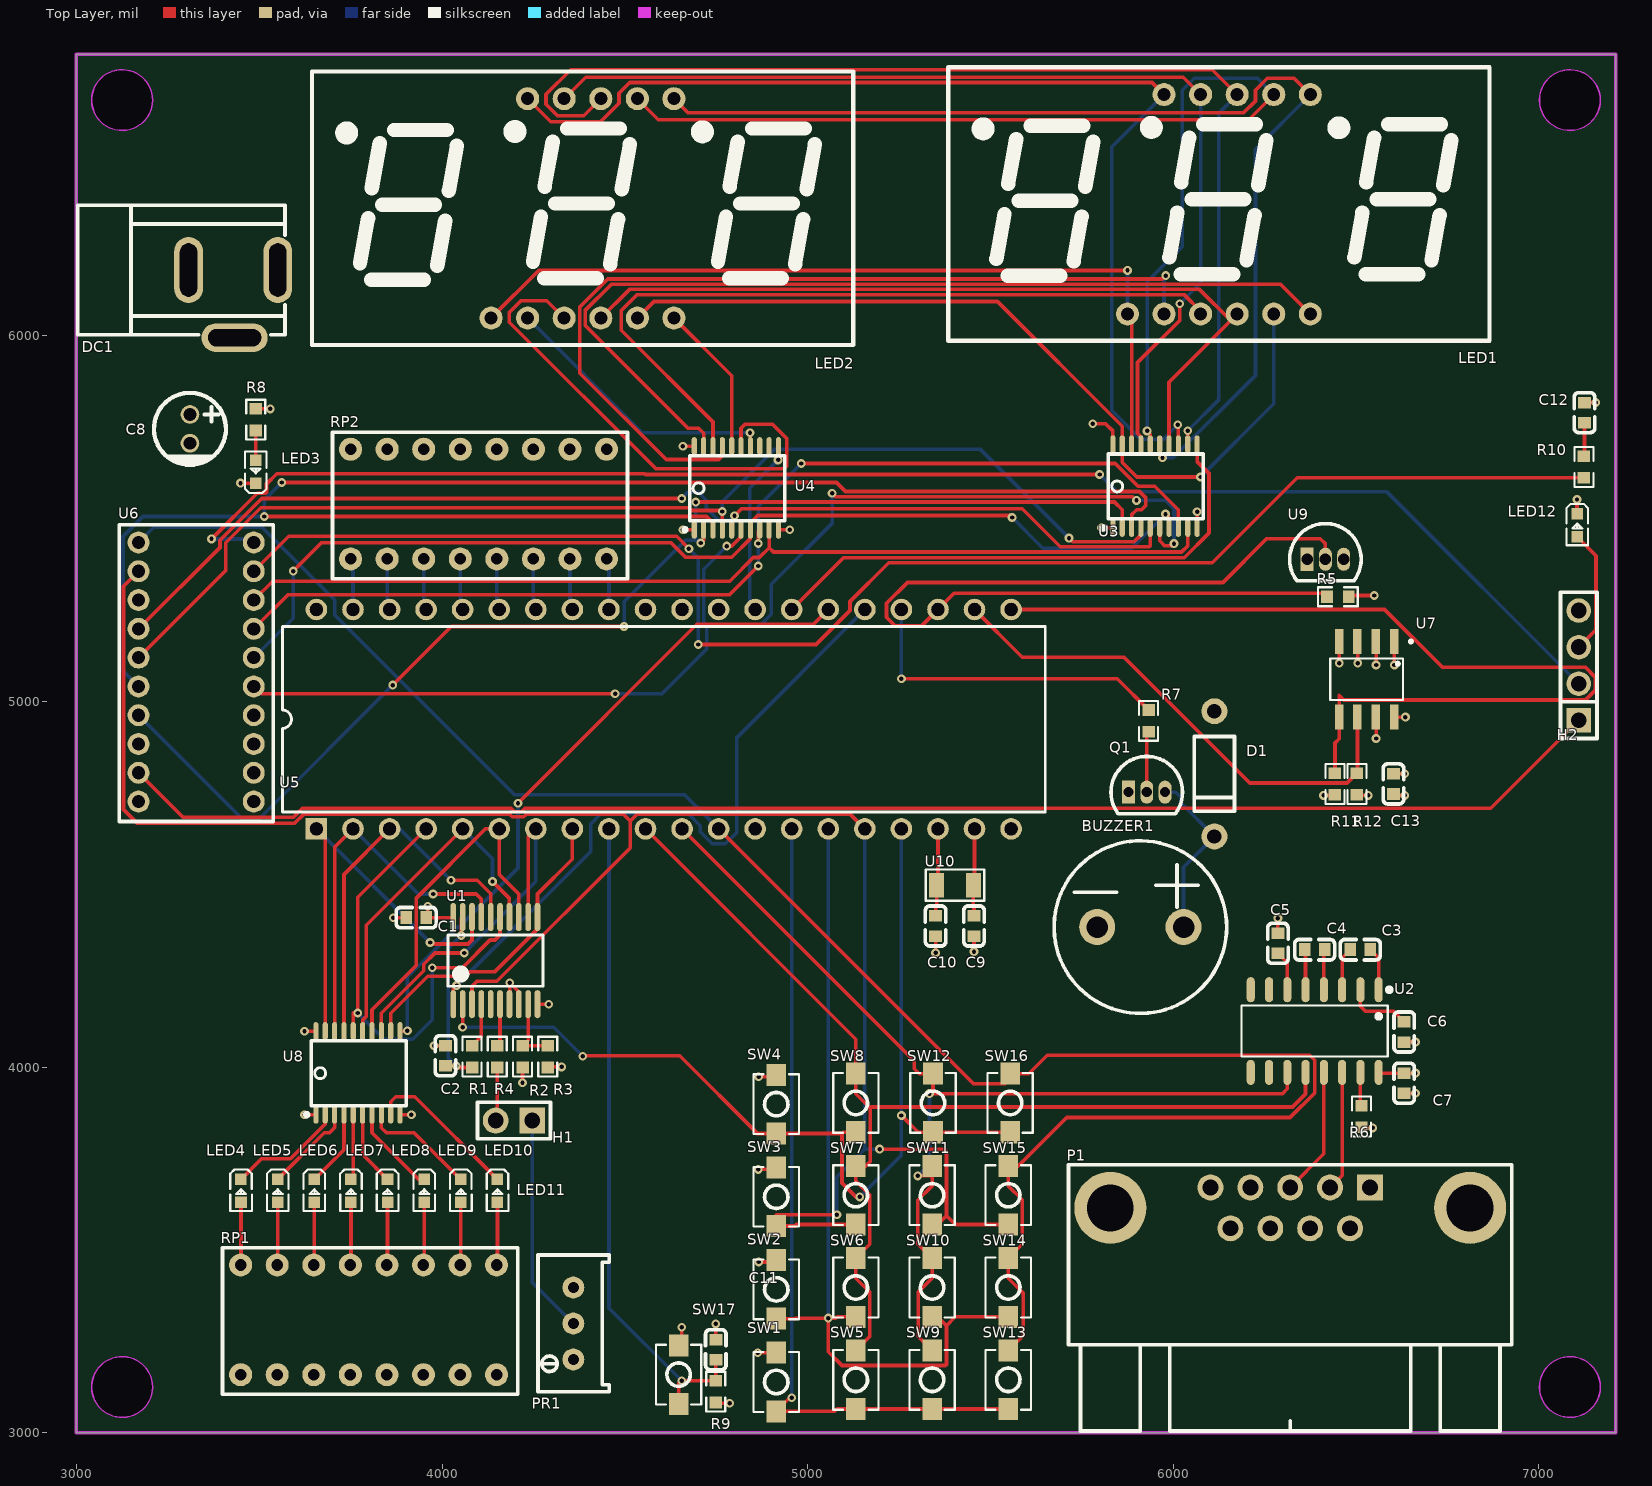
[diagram p0: Top Layer view]
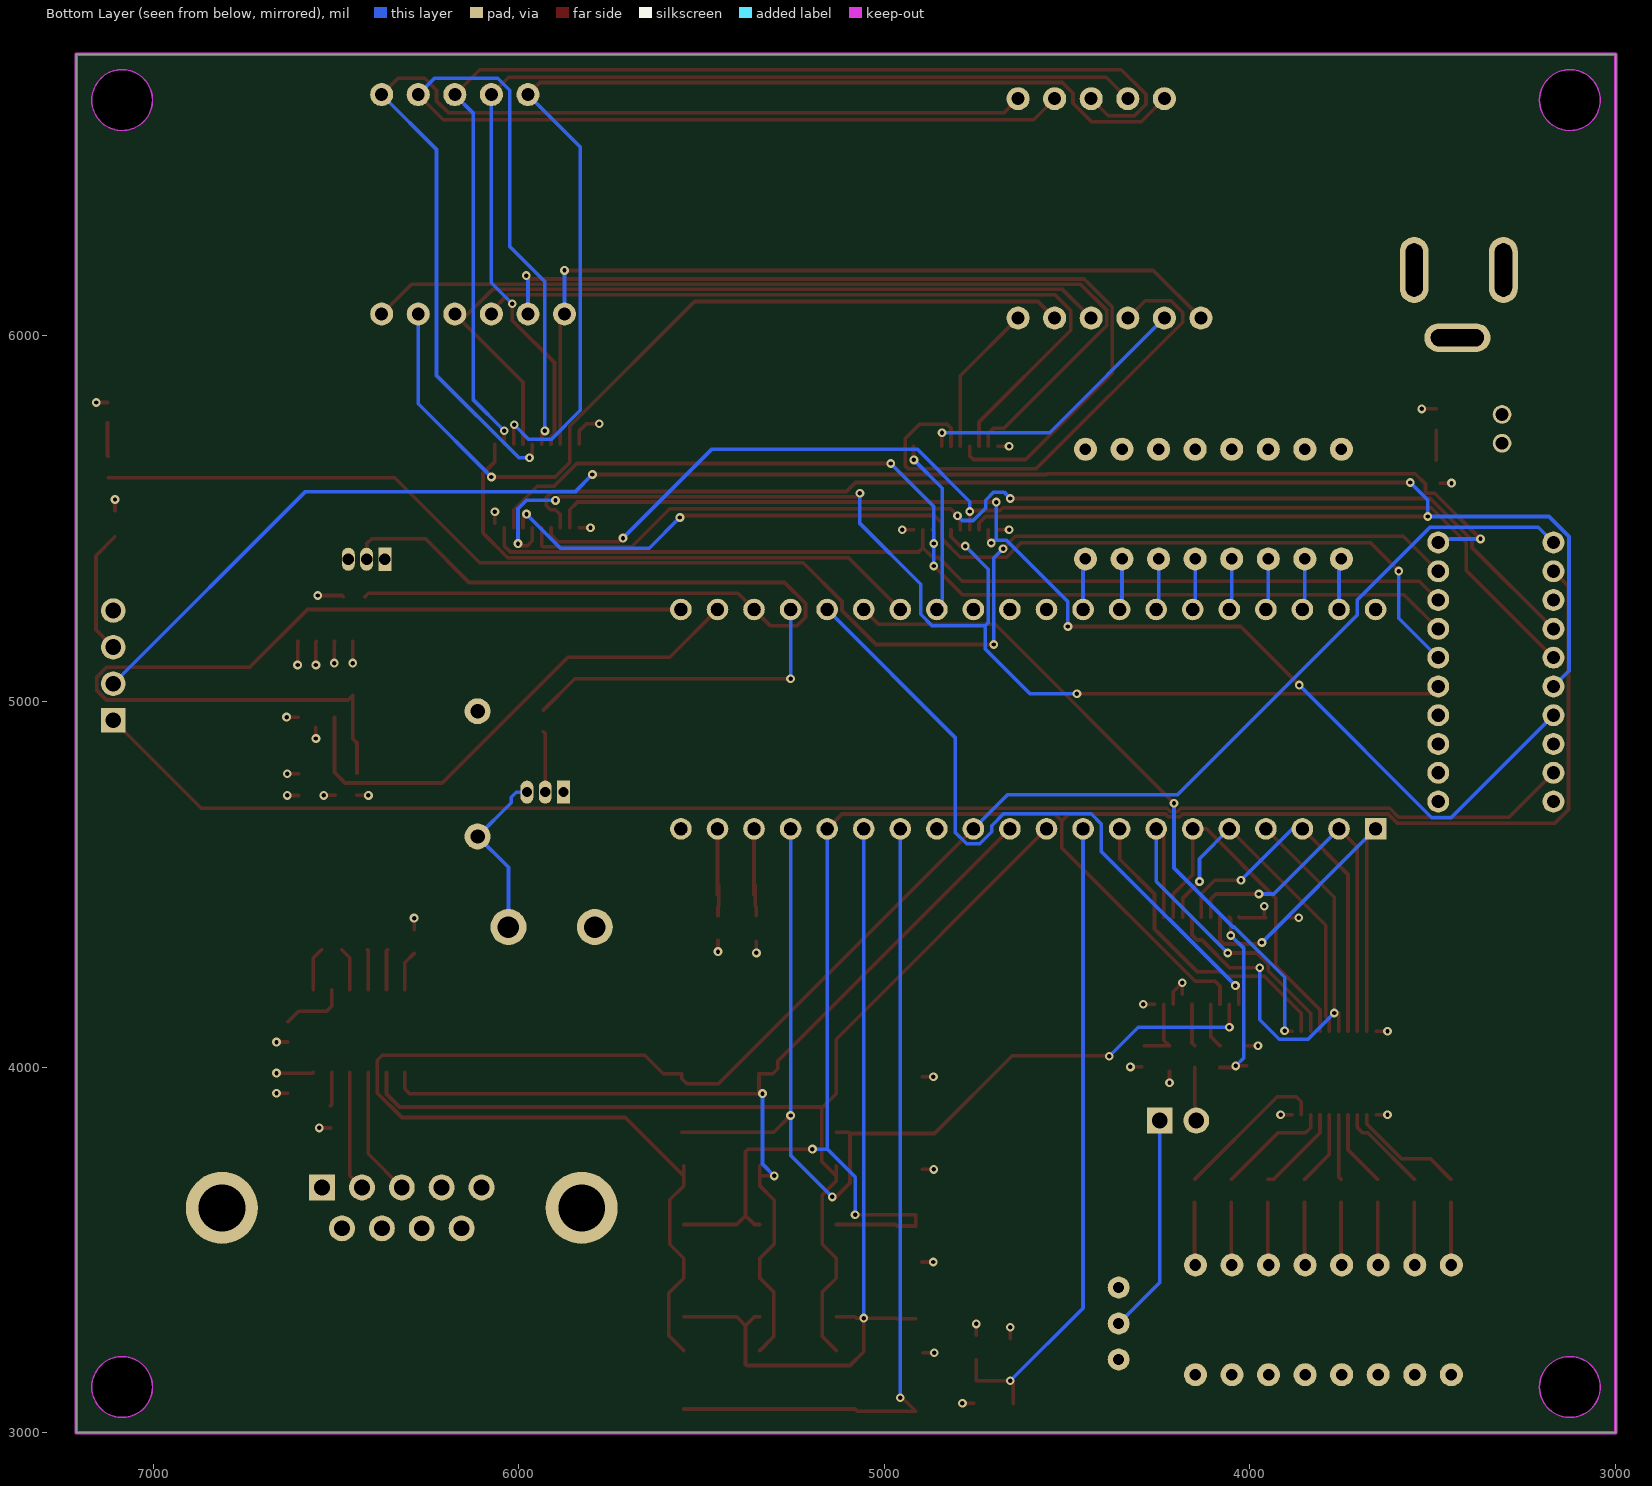
[diagram p1: Bottom Layer view, seen from below]
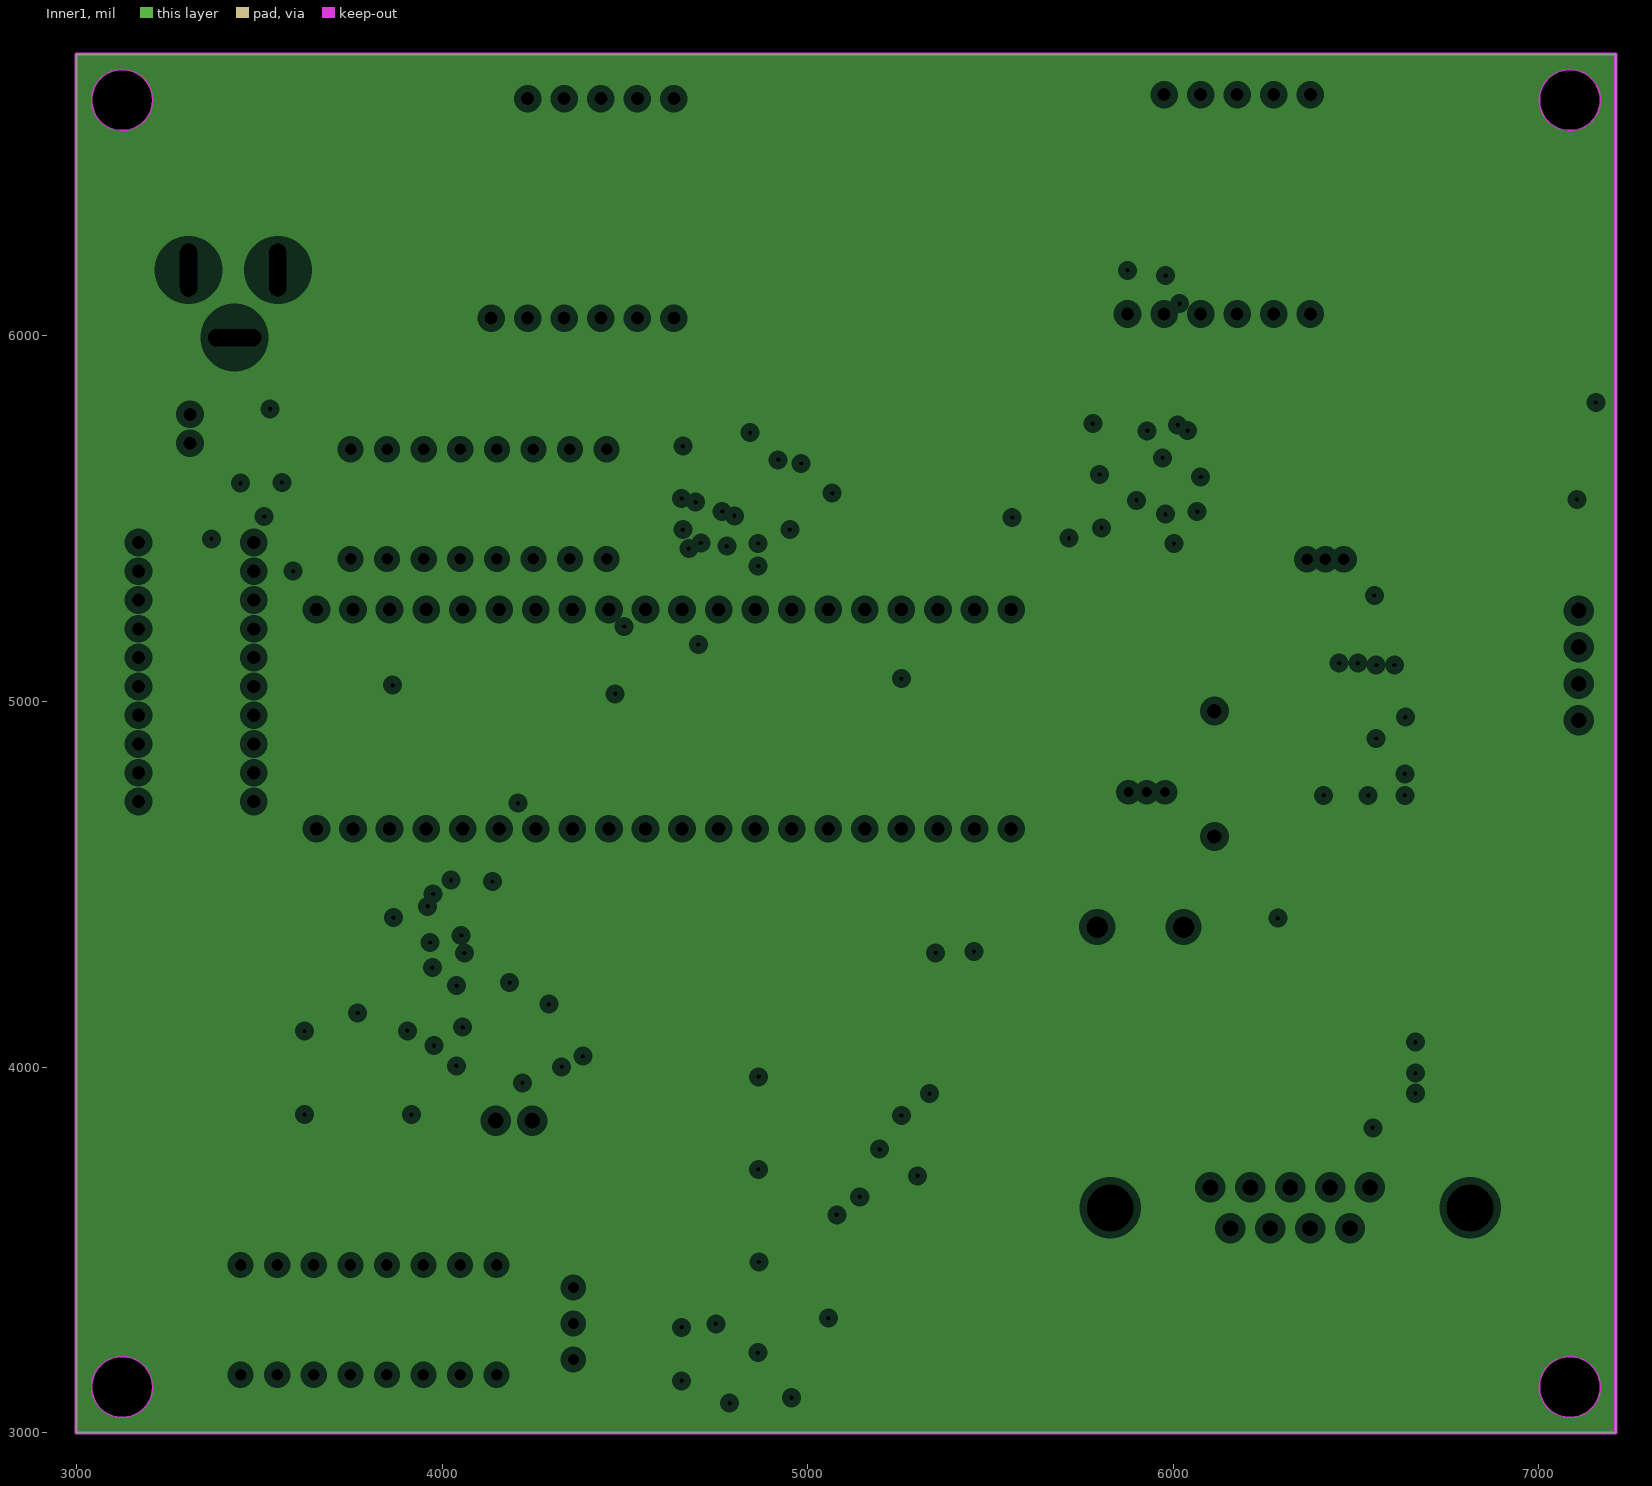
[diagram p2: Inner1, clearances drawn from the general rule]
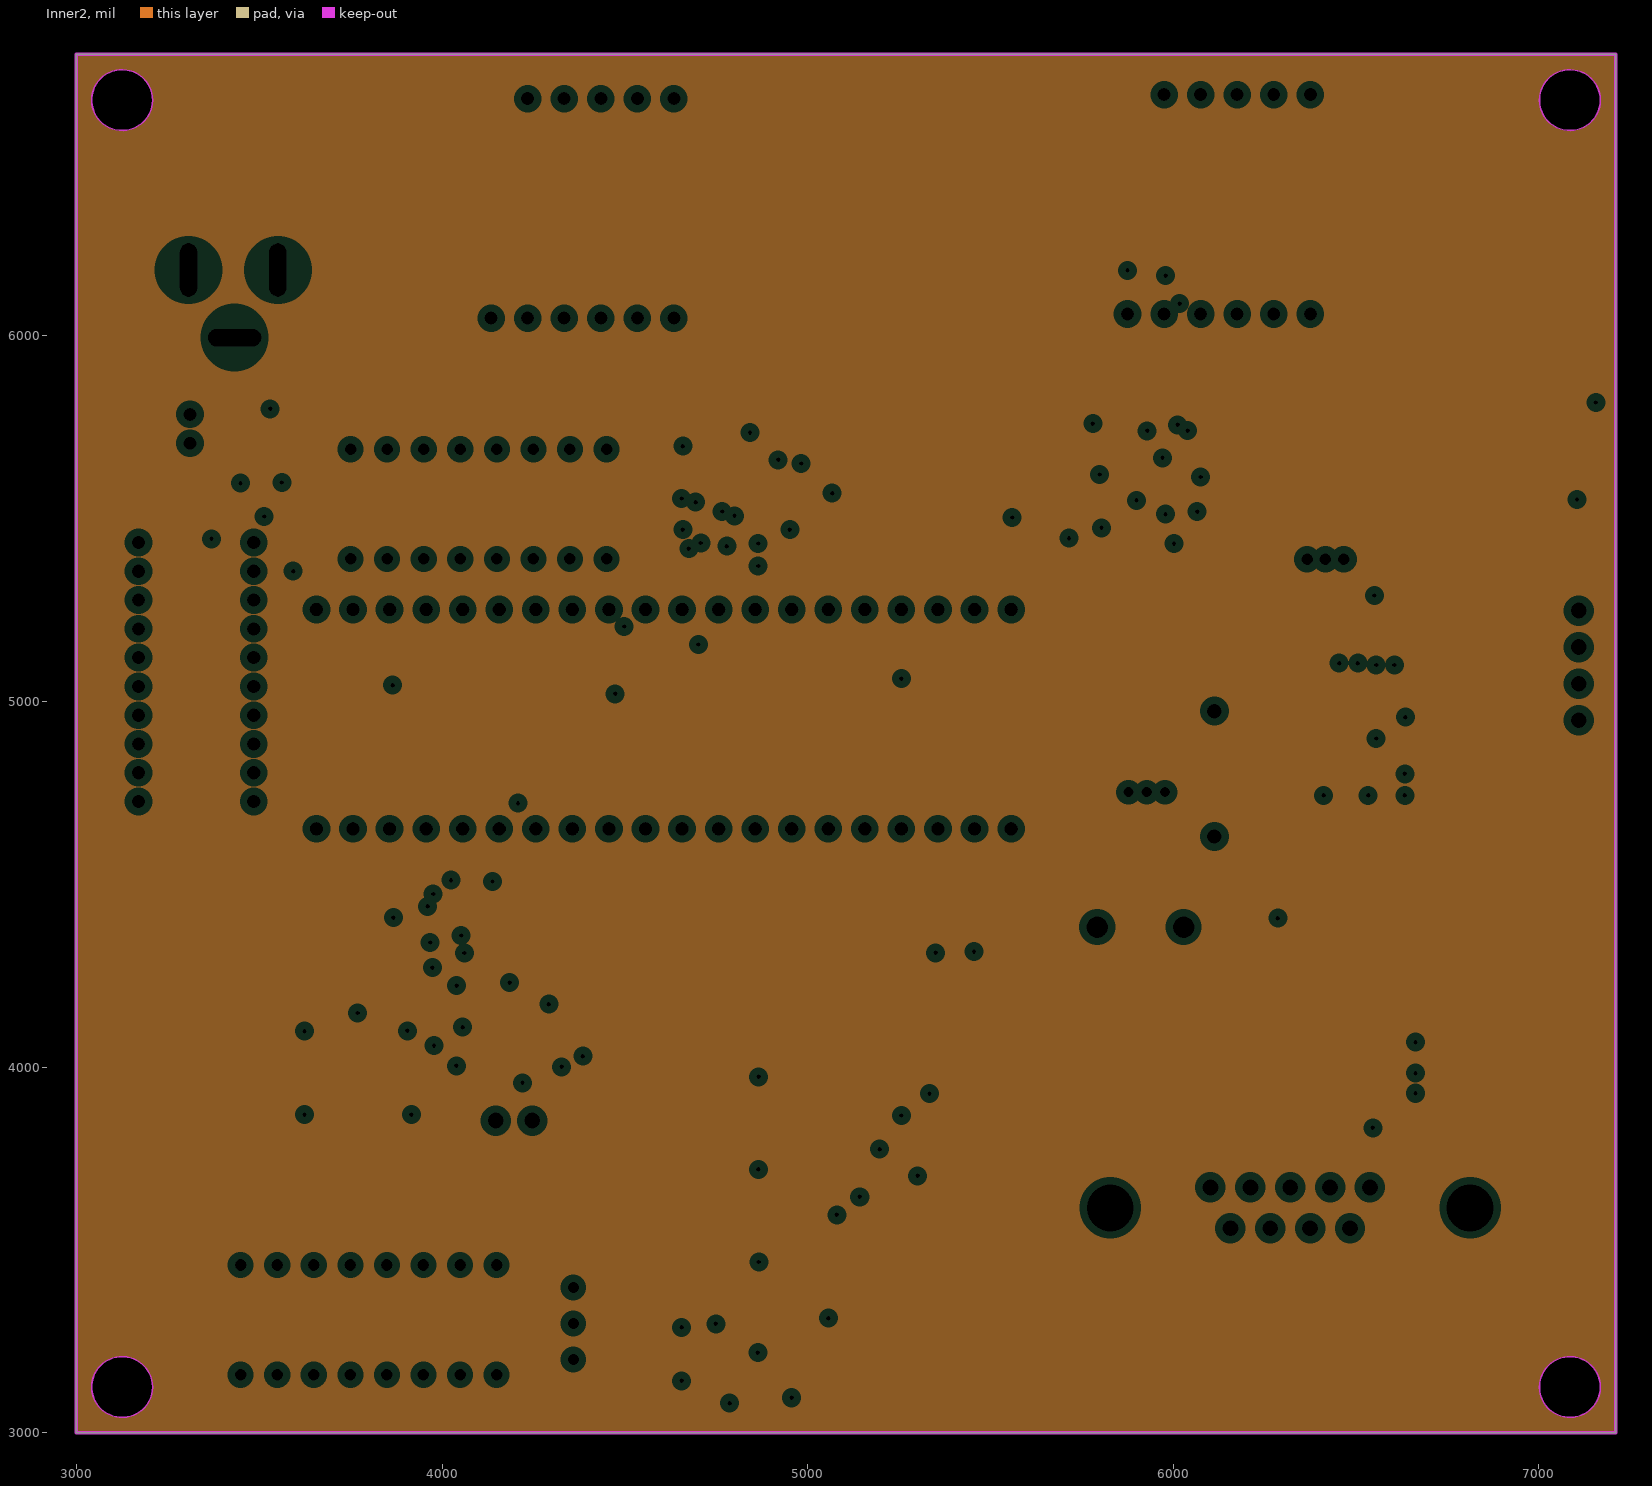
[diagram p3: Inner2, clearances drawn from the general rule]
# Altium PCB MISC49866.pcbdoc (part 1 of 2)
Units mil, origin at the board's own origin, x right, y up, seen from the top; angles counter-clockwise.
Board outline 4210 x 3770 mil, 4 copper layers (Top Layer, Inner1, Inner2, Bottom Layer), stack 62.447 mil thick; 74 components, 100 nets, 357 pads, 104 vias.

## Layer stack, top to bottom
Top Layer: signal copper 1.378
Dielectric1: surface 8.283, 7628 RC49% 8.6mil, Dk 4.4
Inner1: plane copper 0.598
Dielectric2: surface 41.929, 1.1mm H/HOZ Copper, Dk 4.43
Inner2: plane copper 0.598
Dielectric3: surface 8.283, 7628 RC49% 8.6mil, Dk 4.4
Bottom Layer: signal copper 1.378

## Board outline
3000,6770 3000,3000 7210,3000 7210,6770
cut-out: 3208.22,6645 cw(c3125,6645) 3041.78,6645 cw(c3125,6645)
cut-out: 7168.22,6645 cw(c7085,6645) 7001.78,6645 cw(c7085,6645)
cut-out: 7168.22,3125 cw(c7085,3125) 7001.78,3125 cw(c7085,3125)
cut-out: 3208.22,3125 cw(c3125,3125) 3041.78,3125 cw(c3125,3125)

## Design rules (kind name [scope] priority, off if disabled: settings)
BoardOutlineClearance copperThickness2oz_1 [All] p2 off: genericclearance=7.99 ignorepadtopadclearanceinfootprint=FALSE except(0: Arc-SplitContinuation Track-SplitContinuation SMDPad-SplitContinuation THPad-SplitContinuation Via-SplitContinuation Fill-SplitContinuation Region-SplitContinuation Poly-SplitContinuation Text-SplitContinuation Hole-SplitContinuation; 5.98: Arc-CutoutEdge SMDPad-CutoutEdge THPad-CutoutEdge Via-CutoutEdge Fill-CutoutEdge Region-CutoutEdge Text-CutoutEdge; 6.93: Hole-OutlineEdge Hole-CutoutEdge; 10: Poly-OutlineEdge Poly-CutoutEdge; 11.81: Arc-OutlineEdge Track-OutlineEdge SMDPad-OutlineEdge THPad-OutlineEdge Via-OutlineEdge Fill-OutlineEdge Region-OutlineEdge Text-OutlineEdge Track-CutoutEdge)
BoardOutlineClearance copperThickness1oz_1 [All] p4: genericclearance=4.02 ignorepadtopadclearanceinfootprint=FALSE except(0: Arc-SplitContinuation Track-SplitContinuation SMDPad-SplitContinuation THPad-SplitContinuation Via-SplitContinuation Fill-SplitContinuation Region-SplitContinuation Poly-SplitContinuation Text-SplitContinuation Hole-SplitContinuation; 6: SMDPad-CutoutEdge THPad-CutoutEdge Via-CutoutEdge Fill-CutoutEdge Region-CutoutEdge Text-CutoutEdge; 6.93: Hole-OutlineEdge Hole-CutoutEdge; 10: Poly-OutlineEdge Poly-CutoutEdge; 11.8: Arc-OutlineEdge Track-OutlineEdge SMDPad-OutlineEdge THPad-OutlineEdge Via-OutlineEdge Fill-OutlineEdge Region-OutlineEdge Text-OutlineEdge; 11.81: Arc-CutoutEdge Track-CutoutEdge)
Clearance copperThickness2oz [All] p1 off: gap=7.99 ignorepadtopadclearanceinfootprint=FALSE except(5.98: SMDPad-Track SMDPad-SMDPad THPad-Track SMDPad-THPad THPad-THPad Track-Via SMDPad-Via THPad-Via Via-Via Fill-Track Region-Track Fill-SMDPad Region-SMDPad Fill-THPad Region-THPad Fill-Via Region-Via Fill-Fill Fill-Region Region-Region Arc-Track Arc-SMDPad Arc-THPad Arc-Via Fill-Arc Region-Arc Arc-Arc Text-Track SMDPad-Text Text-THPad Text-Via Fill-Text Region-Text Arc-Text Text-Text; 6.93: Hole-Track Hole-SMDPad Hole-THPad Hole-Via Fill-Hole Region-Hole Hole-Arc Hole-Text; 10: Poly-Track Poly-SMDPad Poly-THPad Poly-Via Poly-Fill Poly-Region Poly-Poly Poly-Arc Poly-Text Poly-Hole)
Clearance copperThickness1oz [All] p3: gap=4.02 ignorepadtopadclearanceinfootprint=FALSE except(5.98: SMDPad-Track SMDPad-SMDPad THPad-Track SMDPad-THPad THPad-THPad Track-Via SMDPad-Via THPad-Via Via-Via Fill-Track Region-Track Fill-SMDPad Region-SMDPad Fill-THPad Region-THPad Fill-Via Region-Via Fill-Fill Fill-Region Region-Region; 6: Arc-Track Arc-SMDPad Arc-THPad Arc-Via Fill-Arc Region-Arc Arc-Arc Text-Track SMDPad-Text Text-THPad Text-Via Fill-Text Region-Text Arc-Text Text-Text; 6.93: Hole-Track Hole-SMDPad Hole-THPad Hole-Via Fill-Hole Region-Hole Hole-Arc Hole-Text; 10: Poly-Track Poly-SMDPad Poly-THPad Poly-Via Poly-Fill Poly-Region Poly-Poly Poly-Arc Poly-Text Poly-Hole)
Creepage creepage [All] p1: checkdistance=0 ignoreinternallayers=TRUE applytopolygonpour=TRUE
DiffPairsRouting differentialPair [All] p1: maxlimit=6 minlimit=6 mostfreqgap=6 toplayer_minwidth=5 toplayer_prefwidth=10 toplayer_maxwidth=100 toplayer_mingap=6 toplayer_prefgap=6 toplayer_maxgap=6 bottomlayer_minwidth=5 bottomlayer_prefwidth=10 bottomlayer_maxwidth=100 bottomlayer_mingap=6 bottomlayer_prefgap=6 bottomlayer_maxgap=6 maxuncoupledlength=10
HoleToHoleClearance otherClearance [All] p1: gap=11.81 allowstackedmicrovias=TRUE
Length netLength [All] p1: minlimit=0 maxlimit=0
MatchedLengths netLengthTolerance [All] p1: tolerance=1000
PasteMaskExpansion pasteMaskExpansion [All] p1: expansion=0
PlaneConnect innerPlane [All] p1: planeconnectstyle=Relief reliefexpansion=20 reliefentries=4 reliefconductorwidth=10 reliefairgap=10
PolygonConnect copperRegion [All] p1: connectstyle=Relief reliefconductorwidth=10 reliefentries=4 polygonreliefangle="90 Angle" airgapwidth=10 via.connectstyle=Relief via.reliefconductorwidth=10 via.reliefentries=4 via.polygonreliefangle="90 Angle" via.airgapwidth=10
RoutingVias viaSize [All] p1: holewidth=12.01 width=24.02 viastyle="Through Hole" minholewidth=11.81 minwidth=19.68 maxholewidth=248.03 maxwidth=393.7
SolderMaskExpansion solderMaskExpansion [IsVia] p1: expansion=-1000 istentingtop=TRUE
SolderMaskExpansion solderMaskExpansion [All] p2: expansion=2 istentingtop=FALSE
Width copperThickness2oz_2 [All] p1 off: maxlimit=100 minlimit=8 preferedwidth=10
Width PWR [(InNet('VCC'))] p2: maxlimit=10 minlimit=10 preferedwidth=10 toplayer_minwidth=10 toplayer_maxwidth=100 toplayer_prefwidth=30 bottomlayer_minwidth=10 bottomlayer_maxwidth=100 bottomlayer_prefwidth=30
Width copperThickness1oz_2 [All] p3: maxlimit=10 minlimit=10 preferedwidth=10 toplayer_minwidth=10 toplayer_maxwidth=100 toplayer_prefwidth=10 bottomlayer_minwidth=10 bottomlayer_maxwidth=100 bottomlayer_prefwidth=10

## Components (designator, comment, footprint, x,y, rotation, side; value= is the part's Value field where it differs from the comment)
BUZZER1 "buzzer" BUZ-TH_BD12.0-P6.00-D0.9-RD 5910.16,4383.1 r0 top
C1 "104" C0603 3929.27,4408.78 r180 top
C2 "104" C0603 4009.27,4030.97 r90 top
C3 "104" C0603 6511.76,4321.11 r180 top
C4 "104" C0603 6386.76,4321.11 r180 top
C5 "104" C0603 6286.36,4338.55 r270 top
C6 "104" C0603 6631.76,4096.11 r90 top
C7 "104" C0603 6631.76,3956.11 r90 top
C8 "100uF" CAP-TH_BD5.0-P2.00-D0.8-FD-10UF50VC110GL 3310.61,5745.83 r270 top
C9 "20PF" C0603 5455.03,4386.04 r90 top
C10 "20PF" C0603 5350.03,4386.04 r90 top
C11 "10uF" C0603 4748.84,3227.23 r90 top
C12 "104" C0603 7124.88,5790.25 r90 top
C13 "104" C0603 6602.32,4774.62 r270 top
D1 "" DO_1N4007 6112.67,4802.17 r90 top
DC1 "" DC-005_2.5 3423.86,6167.74 r180 top
H1 "" HDR-TH_2P-P2.54-V-M-1 4196.93,3853.78 r180 top
H2 "" HDR-TH_4P-P2.54-V-M 7109.27,5098.78 r90 top
LED1 "3631BS" LED-SEG-TH_11P-L37.5-W19.0-P2.54-LS15.2-BL_1 6125,6360 r180 top
LED2 "3631BS" LED-SEG-TH_11P-L37.5-W19.0-P2.54-LS15.2-BL_1 4384.27,6348.78 r180 top
LED3 "" LED_0603 3490.61,5630.83 r90 top
LED4 "" LED_0603 3450.42,3659.36 r270 top
LED5 "" LED_0603 3550.64,3659.36 r270 top
LED6 "" LED_0603 3650.86,3659.36 r270 top
LED7 "" LED_0603 3751.08,3659.36 r270 top
LED8 "" LED_0603 3851.3,3659.36 r270 top
LED9 "" LED_0603 3951.52,3659.36 r270 top
LED10 "" LED_0603 4051.73,3659.36 r270 top
LED11 "" LED_0603 4151.95,3659.36 r270 top
LED12 "" LED_0603 7105,5480 r270 top
P1 "DB9FL" DB9-TH_DB9F 6320,3615 r0 top
PR1 "10kΩ" R_3296 4354.27,3298.78 r90 top
Q1 "" S8550P_TO-92 5927.67,4752.17 r0 top
R1 "10K" R0603 4082.23,4028.78 r90 top
R2 "1K" R0603 4220.26,4028.78 r270 top
R3 "1K" R0603 4289.27,4028.78 r90 top
R4 "510K" R0603 4151.25,4028.78 r90 top
R5 "4.7K" R0603 6450.25,5286.78 r0 top
R6 "0" R0603 6515,3865 r90 top
R7 "2K" R0603 5932.67,4947.17 r270 top
R8 "1K" R0603 3490.61,5770.83 r90 top
R9 "10K" R0603 4748.84,3112.23 r90 top
R10 "0" R0603 7123.25,5641.69 r90 top
R11 "4.7K" R0603 6442.32,4774.62 r270 top
R12 "4.7K" R0603 6502.32,4774.62 r270 top
RP1 "" DIP-16_L20.3-W10.2-P2.54-LS7.6-BL 3799.27,3308.78 r0 top
RP2 "" DIP-16_L20.3-W10.2-P2.54-LS7.6-BL 4100,5540 r0 top
SW1 "" Key_SMD_3x4x2 4914.27,3138.78 r270 top
SW2 "" Key_SMD_3x4x2 4914.27,3392.12 r270 top
SW3 "" Key_SMD_3x4x2 4914.27,3645.45 r270 top
SW4 "" Key_SMD_3x4x2 4914.27,3898.78 r270 top
SW5 "" Key_SMD_3x4x2 5131.95,3144.87 r90 top
SW6 "" Key_SMD_3x4x2 5131.95,3397.24 r90 top
SW7 "" Key_SMD_3x4x2 5131.95,3649.62 r90 top
SW8 "" Key_SMD_3x4x2 5131.95,3901.99 r90 top
SW9 "" Key_SMD_3x4x2 5340.44,3144.87 r90 top
SW10 "" Key_SMD_3x4x2 5340.44,3397.24 r90 top
SW11 "" Key_SMD_3x4x2 5340.44,3649.62 r90 top
SW12 "" Key_SMD_3x4x2 5342.94,3901.99 r90 top
SW13 "" Key_SMD_3x4x2 5548.93,3144.87 r90 top
SW14 "" Key_SMD_3x4x2 5548.93,3397.24 r90 top
SW15 "" Key_SMD_3x4x2 5548.93,3649.62 r90 top
SW16 "" Key_SMD_3x4x2 5553.93,3901.99 r90 top
SW17 "" Key_SMD_3x4x2 4647.12,3159.02 r270 top
U1 "ADC0804CN" ADC0804CN 4131,4303.28 r0 top
U2 "MAX232ESE" MAX232ESE 6591.76,4211.11 r180 top
U3 "MC74HC573DW" MC74HC573DW 5835,5475 r90 top
U4 "MC74HC573DW" MC74HC573DW 4690,5470 r90 top
U5 "P89C51RC2HBP" P89C51RC23N_01 4754.31,4907.16 r0 top
U6 "DAC0832LCJ" DAC0832LCJ 3485,5435 r0 top
U7 "AT24C02" SOIC-8_L5.0-W4.0-P1.27-LS6.2-TL 6528.96,5060.68 r270 top
U8 "MC74HC573DW" MC74HC573DW 3655,3870 r90 top
U9 "DS18B20" TO-92-3_L4.9-W3.7-P1.27-L 6416.26,5389.12 r0 top
U10 "32768/10ppm/12.5pF" osc-smd_l3.2-w1.5 5403.24,4497.68 r0 top

## Footprints (in the part's own frame and the unit in brackets; to place one, negate y for a bottom-side part, rotate by r counter-clockwise, add the part's x,y. Pads: shape width x height; smd on the part's side, far side on the other; paste and mask are expansions set on the pad)
ADC0804CN [mm]
  oval 0.4x1.95 smd: 1(-2.544,-3.334) 2(-1.894,-3.334) 3(-1.244,-3.334) 4(-0.594,-3.334) 5(0.056,-3.334) 6(0.706,-3.334) 7(1.356,-3.334) 8(2.006,-3.334) 9(2.656,-3.334) 10(3.306,-3.334) 11(3.306,2.724) 12(2.656,2.724) 13(2.006,2.724) 14(1.356,2.724) 15(0.706,2.724) 16(0.056,2.724) 17(-0.594,2.724) 18(-1.244,2.724) 19(-1.894,2.724) 20(-2.544,2.724)
  silkscreen extent -2.92,-2.08 3.68,1.47
BUZ-TH_BD12.0-P6.00-D0.9-RD [mm]
  round 2.5 hole 1.5 paste+0 mask+0.05: 1(-3,0) 2(3,0)
  silkscreen extent -5.99,-5.99 5.99,5.99
C0603 [mm]
  rect 0.8x0.9 smd: 1(-0.7,0) 2(0.7,0)
  silkscreen extent -1.39,-0.71 1.39,0.71
CAP-TH_BD5.0-P2.00-D0.8-FD-10UF50VC110GL [mm]
  round 1.3 hole 0.9 paste+0 mask+0.051: 1(-1,0) 2(1,0)
  silkscreen extent -2.5,-2.5 2.5,2.5
DAC0832LCJ [mil]
  round 60 hole 36 paste+0 mask+2: 1(-314.96,0) 2(-314.96,-78.74) 3(-314.96,-157.48) 4(-314.96,-236.22) 5(-314.96,-314.96) 6(-314.96,-393.7) 7(-314.96,-472.44) 8(-314.96,-551.18) 9(-314.96,-629.92) 10(-314.96,-708.66) 11(0,0) 12(0,-78.74) 13(0,-157.48) 14(0,-236.22) 15(0,-314.96) 16(0,-393.7) 17(0,-472.44) 18(0,-551.18) 19(0,-629.92) 20(0,-708.66)
  silkscreen extent -368,-763 53,49
DB9-TH_DB9F [mm]
  rect 1.8x1.8 hole 1.1: 1(5.54,1.42)
  round 1.8 hole 1.1: 2(2.77,1.42) 3(0,1.42) 4(-2.77,1.42) 5(-5.54,1.42) 6(4.155,-1.42) 7(1.385,-1.42) 8(-1.385,-1.42) 9(-4.155,-1.42)
  round 5 hole 3.25: 10(-12.5,0) 11(12.5,0)
  silkscreen extent -15.4,-15.5 15.4,3
DC-005_2.5 [mm]
  oval 2x4.6 hole 1.2 slot 3.7 at 90 deg paste+0 mask+0.051: 1(-3.227,-0.318) 2(2.973,-0.318)
  oval 4.6x2 hole 1.2 slot 3.7 at 0 deg paste+0 mask+0.051: 3(-0.227,4.382)
  silkscreen extent -3.73,-4.82 10.67,4.18
DIP-16_L20.3-W10.2-P2.54-LS7.6-BL [mm]
  round 1.6 hole 0.8: 1(-8.89,-3.81) 2(-6.35,-3.81) 3(-3.81,-3.81) 4(-1.27,-3.81) 5(1.27,-3.81) 6(3.81,-3.81) 7(6.35,-3.81) 8(8.89,-3.81) 9(8.89,3.81) 10(6.35,3.81) 11(3.81,3.81) 12(1.27,3.81) 13(-1.27,3.81) 14(-3.81,3.81) 15(-6.35,3.81) 16(-8.89,3.81)
  silkscreen extent -10.15,-5.18 10.35,5
DO_1N4007 [mm]
  round 1.8 hole 1 paste+0 mask+0.051: 1(-4.35,0) 2(4.35,0)
  silkscreen extent -2.6,-1.4 2.6,1.4
HDR-TH_2P-P2.54-V-M-1 [mm]
  rect 1.8x1.8 hole 1.1: 1(-1.27,0)
  round 1.8 hole 1.1: 2(1.27,0)
  silkscreen extent -2.54,-1.27 2.54,1.27
HDR-TH_4P-P2.54-V-M [mm]
  rect 1.7x1.7 hole 1.1: 1(-3.81,0)
  round 1.7 hole 1.1: 2(-1.27,0) 3(1.27,0) 4(3.81,0)
  silkscreen extent -5.08,-1.27 5.08,1.27
Key_SMD_3x4x2 [mm]
  rect 1.53x1.36 smd paste+0 mask+0.051: 1(-2.035,0) 2(2.035,0)
  silkscreen extent -2.08,-1.58 2.08,1.58
LED-SEG-TH_11P-L37.5-W19.0-P2.54-LS15.2-BL_1 [mm]
  round 1.6 hole 0.9: 1(-6.35,-7.62) 2(-3.81,-7.62) 3(-1.27,-7.62) 4(1.27,-7.62) 5(3.81,-7.62) 7(6.35,7.62) 8(3.81,7.62) 9(1.27,7.62) 10(-1.27,7.62) 11(-3.81,7.62) 12(-6.35,7.62)
  silkscreen extent -18.8,-9.51 18.8,9.49
LED_0603 [mil]
  rect 31.5x31.5 smd paste+0 mask+2: 1(-33.5,-0.4) 2(29.5,-0.2)
  silkscreen extent -61,-30 53,30
MAX232ESE [mm]
  oval 0.56x1.745 smd paste+0.102 mask+0.051: 1(0.755,-0.016) 2(2.025,-0.016) 3(3.295,-0.016) 4(4.565,-0.016) 5(5.835,-0.016) 6(7.105,-0.016) 7(8.375,-0.016) 8(9.645,-0.016) 9(9.645,5.728) 10(8.375,5.728) 11(7.105,5.728) 12(5.835,5.728) 13(4.565,5.728) 14(3.295,5.728) 15(2.025,5.728) 16(0.755,5.728)
  silkscreen extent -0.13,-0.17 10.28,4.63
MC74HC573DW [mm]
  oval 1.26x0.36 smd: 1(0,0) 2(0,-0.65) 3(0,-1.3) 4(0,-1.95) 5(0,-2.6) 6(0,-3.25) 7(0,-3.9) 8(0,-4.55) 9(0,-5.2) 10(0,-5.85) 11(5.8,-5.85) 12(5.8,-5.2) 13(5.8,-4.55) 14(5.8,-3.9) 15(5.8,-3.25) 16(5.8,-2.6) 17(5.8,-1.95) 18(5.8,-1.3) 19(5.8,-0.65) 20(5.8,0)
  silkscreen extent -0.05,-6.27 5.13,0.68
osc-smd_l3.2-w1.5 [mm]
  rect 1.05x1.7 smd: 1(-1.275,0) 2(1.275,0)
  silkscreen extent -2.03,-1.08 2.03,1.08
P89C51RC23N_01 [mm]
  rect 1.5x1.5 hole 0.9 slot 0.905 at 90 deg paste+0 mask+0.051: 1(-27.883,-6.489)
  round 1.5 hole 0.9 slot 0.905 at 90 deg paste+0 mask+0.051: 2(-25.343,-6.489) 3(-22.803,-6.489) 4(-20.263,-6.489) 5(-17.723,-6.489) 6(-15.183,-6.489) 7(-12.643,-6.489) 8(-10.103,-6.489) 9(-7.563,-6.489) 10(-5.023,-6.489) 11(-2.483,-6.489) 12(0.057,-6.489) 13(2.597,-6.489) 14(5.137,-6.489) 15(7.677,-6.489) 16(10.217,-6.489) 17(12.757,-6.489) 18(15.297,-6.489) 19(17.837,-6.489) 20(20.377,-6.489) 21(20.377,8.751) 22(17.837,8.751) 23(15.297,8.751) 24(12.757,8.751) 25(10.217,8.751) 26(7.677,8.751) 27(5.137,8.751) 28(2.597,8.751) 29(0.057,8.751) 30(-2.483,8.751) 31(-5.023,8.751) 32(-7.563,8.751) 33(-10.103,8.751) 34(-12.643,8.751) 35(-15.183,8.751) 36(-17.723,8.751) 37(-20.263,8.751) 38(-22.803,8.751) 39(-25.343,8.751) 40(-27.883,8.751)
  silkscreen extent -30.25,-5.32 22.75,7.58
R0603 [mil]
  rect 31.75x34.02 smd paste-3937.01 mask+2: 1(-29.66,0) 2(29.66,0)
  silkscreen extent -55,-26 55,26
R_3296 [mil]
  round 60 hole 30 paste+0 mask+2: 1(-98.4,-5) 2(0,-5) 3(98.4,-5)
  silkscreen extent -187,-103 187,92
S8550P_TO-92 [mm]
  rect 0.9x1.6 hole 0.7 paste+0 mask+0.051: 1(-1.27,0)
  oval 0.9x1.6 hole 0.7 paste+0 mask+0.051: 2(0,0) 3(1.27,0)
  silkscreen extent -2.48,-1.5 2.48,2.48
SOIC-8_L5.0-W4.0-P1.27-LS6.2-TL [mil]
  rect 68.92x23.18 smd: 1(-103.36,75) 2(-103.36,25) 3(-103.36,-25) 4(-103.36,-75) 5(103.36,-75) 6(103.36,-25) 7(103.36,25) 8(103.36,75)
  silkscreen extent -107,-99 57,125
TO-92-3_L4.9-W3.7-P1.27-L [mm]
  rect 0.9x1.6 hole 0.8: 1(-1.27,0)
  oval 0.9x1.6 hole 0.8: 2(0,0) 3(1.27,0)
  silkscreen extent -2.48,-1.5 2.48,2.48

## Via types
v1: diameter 24.02, hole 12, Top Layer to Bottom Layer, 104 vias

## Nets (pads, with @x,y where several pads share a name; then routed paths per layer and width w, separated by ;. In a path a pad name is that pad's centre, name@x,y a point inside that pad or via, vN(x,y) a via of type N, cw(c..) or ccw(c..) an arc to the next point about the centre after c; other vN are vias at no path point)
18B20: R5.1 U5.23 U9.2 | length 2613.9
  Top Layer w10: U9.2@6416.26,5389.12 6416.26,5431.36 6402.49,5445.13 6255.24,5445.13 6135.86,5325.75 5273.08,5325.75 5215.87,5268.54 5215.87,5230.52 5238.67,5207.72 5312.59,5207.72 U5.23@5356.56,5251.69 5400.67,5295.8 6411.57,5295.8 R5.1@6420.59,5286.78
$1N14: R1.2 U1.4 | length 124.1
  Top Layer w10: R1.2@4082.23,4058.44 4107.62,4083.82 U1.4@4107.62,4172.03
$1N15: C2.1 R1.1 U1.19 | length 507.6
  Top Layer w10: C2.1@4009.27,4003.41 v1(4039.19,4003.41) 4043.48,3999.12 R1.1@4082.23,3999.12 ; v1(4052.37,4359.97) 4052.37,4406.46 U1.19@4056.44,4410.54
  Bottom Layer w10: v1(4039.19,4003.41) 4016.71,4025.89 4016.71,4324.31 v1(4052.37,4359.97)
$1N18: H1.1 PR1.2 | length 601.5
  Bottom Layer w10: H1.1@4246.93,3853.78 4246.93,3411.12 PR1.2@4359.27,3298.78
$1N20: R2.1 R3.2 U1.9 | length 189
  Top Layer w10: U1.9@4235.57,4172.03 4235.57,4073.76 R2.1@4220.26,4058.44 R3.2@4289.27,4058.44
$1N23: R4.2 U1.6 | length 116.7
  Top Layer w10: R4.2@4151.25,4058.44 4158.81,4066 U1.6@4158.8,4172.03
$1N24: H1.2 R4.1 | length 147.1
  Top Layer w10: H1.2@4146.93,3853.78 4151.25,3858.09 R4.1@4151.25,3999.12
$1N28: C3.1 U2.1 | length 118.8
  Top Layer w10: C3.1@6539.32,4321.11 6562.02,4298.41 U2.1@6562.02,4211.76
$1N29: C3.2 U2.3 | length 118.5
  Top Layer w10: U2.3@6462.02,4211.76 6462.02,4298.93 C3.2@6484.2,4321.11
$1N30: C4.2 U2.5 | length 110.5
  Top Layer w10: C4.2@6359.2,4321.11 6362.02,4318.29 U2.5@6362.02,4211.76
$1N31: C4.1 U2.4 | length 110.3
  Top Layer w10: U2.4@6412.02,4211.76 6412.02,4318.81 C4.1@6414.32,4321.11
$1N34: R6.2 U2.15 | length 92.2
  Top Layer w10: U2.15@6512.02,3985.58 6512.02,3897.64 R6.2@6515,3894.66
$1N36: P1.3 U2.13 | length 352.8
  Top Layer w10: P1.3@6320.01,3670.91 6412.02,3762.93 U2.13@6412.02,3985.58
$1N37: P1.2 U2.14 | length 328.3
  Top Layer w10: P1.2@6429.06,3670.91 6462.02,3703.87 U2.14@6462.02,3985.58
$1N38: C5.2 U2.6 | length 109.9
  Top Layer w10: C5.2@6286.35,4310.99 6312.02,4285.32 U2.6@6312.02,4211.76
$1N40: C6.2 U2.2 | length 182.6
  Top Layer w10: U2.2@6512.02,4211.76 6512.02,4166.68 6525.79,4152.91 6602.52,4152.91 C6.2@6631.76,4123.67
$1N109: BUZZER1.2 D1.1 Q1.3 | length 476.9
  Bottom Layer w10: Q1.3@5977.67,4752.17 6006.62,4752.17 6020.39,4738.4 6020.39,4723.19 D1.1@6112.67,4630.91 6028.28,4546.52 BUZZER1.2@6028.27,4383.1
$1N111: Q1.2 R7.2 | length 167.4
  Top Layer w10: Q1.2@5927.67,4752.17 5927.67,4912.51 R7.2@5932.67,4917.51
$1N114: LED3.2 R8.1 | length 80.9
  Top Layer w10: R8.1@3490.61,5741.17 3490.81,5740.96 LED3.2@3490.81,5660.33
$1N128: LED4.1 U8.2 | length 318.8
  Top Layer w10: LED4.1@3450.02,3692.86 3506.48,3749.31 3585.34,3749.31 3680.59,3844.56 U8.2@3680.59,3870
$1N129: LED5.1 U8.3 | length 250.1
  Top Layer w10: LED5.1@3550.24,3692.86 3678.08,3820.7 3692.41,3820.7 3706.18,3834.47 U8.3@3706.18,3870
$1N130: LED5.2 RP1.15 | length 171.6
  Top Layer w10: RP1.15@3549.27,3458.78 3550.44,3459.94 LED5.2@3550.44,3629.86
$1N131: LED7.2 RP1.13 | length 171.7
  Top Layer w10: RP1.13@3749.27,3458.78 3750.88,3460.38 LED7.2@3750.88,3629.86
$1N132: LED7.1 U8.5 | length 179.9
  Top Layer w10: LED7.1@3750.68,3692.86 3757.36,3699.54 U8.5@3757.36,3870
$1N133: LED6.1 U8.4 | length 210.8
  Top Layer w10: LED6.1@3650.46,3692.86 3731.77,3774.17 U8.4@3731.77,3870
$1N134: LED9.2 RP1.11 | length 171.9
  Top Layer w10: RP1.11@3949.27,3458.78 3951.32,3460.82 LED9.2@3951.32,3629.86
$1N135: LED9.1 U8.7 | length 244.8
  Top Layer w10: U8.7@3808.54,3870 3808.54,3820.7 3936.38,3692.86 LED9.1@3951.12,3692.86
$1N136: LED8.1 U8.6 | length 205.3
  Top Layer w10: U8.6@3782.95,3870 3782.95,3760.81 LED8.1@3850.9,3692.86
$1N137: LED11.2 RP1.9 | length 172.1
  Top Layer w10: RP1.9@4149.27,3458.78 4151.76,3461.26 LED11.2@4151.75,3629.86
$1N138: LED11.1 U8.9 | length 426.9
  Top Layer w10: U8.9@3859.72,3870 3859.72,3905.53 3873.49,3919.3 3925.12,3919.3 LED11.1@4151.55,3692.86
$1N139: LED10.1 U8.8 | length 311.4
  Top Layer w10: U8.8@3834.13,3870 3834.13,3834.47 3847.9,3820.7 3923.5,3820.7 LED10.1@4051.33,3692.86
$1N140: LED4.2 RP1.16 | length 171.5
  Top Layer w10: RP1.16@3449.27,3458.78 3450.23,3459.73 LED4.2@3450.22,3629.86
$1N141: LED6.2 RP1.14 | length 171.7
  Top Layer w10: RP1.14@3649.27,3458.78 3650.66,3460.16 LED6.2@3650.66,3629.86
$1N142: LED8.2 RP1.12 | length 171.8
  Top Layer w10: RP1.12@3849.27,3458.78 3851.1,3460.6 LED8.2@3851.1,3629.86
$1N143: LED10.2 RP1.10 | length 172
  Top Layer w10: RP1.10@4049.27,3458.78 4051.54,3461.04 LED10.2@4051.53,3629.86
$1N162: RP2.8 U5.32 | length 141
  Bottom Layer w10: RP2.8@4450,5390 4456.55,5383.44 U5.32@4456.56,5251.69
$1N163: RP2.7 U5.33 | length 141
  Bottom Layer w10: RP2.7@4350,5390 4349.99,5258.25 U5.33@4356.56,5251.69
$1N164: RP2.6 U5.34 | length 141
  Bottom Layer w10: RP2.6@4250,5390 4249.99,5258.25 U5.34@4256.56,5251.69
$1N165: RP2.5 U5.35 | length 141
  Bottom Layer w10: RP2.5@4150,5390 4150,5258.25 U5.35@4156.56,5251.69
$1N166: RP2.4 U5.36 | length 141
  Bottom Layer w10: RP2.4@4050,5390 4050,5258.25 U5.36@4056.56,5251.69
$1N167: RP2.3 U5.37 | length 141
  Bottom Layer w10: RP2.3@3950,5390 3950,5258.25 U5.37@3956.56,5251.69
$1N168: RP2.2 U5.38 | length 141
  Bottom Layer w10: RP2.2@3850,5390 3850,5258.25 U5.38@3856.56,5251.69
$1N169: RP2.1 U5.39 | length 141
  Bottom Layer w10: RP2.1@3750,5390 3756.56,5383.44 U5.39@3756.56,5251.69
$1N205: C12.1 R10.2 | length 92
  Top Layer w10: R10.2@7123.25,5671.35 7124.88,5672.97 C12.1@7124.88,5762.69
$1N206: R10.1 U6.12 | length 4142.1
  Top Layer w10: U6.12@3485,5356.26 3580.48,5451.74 4641.75,5451.74 v1(4675.38,5418.11) ; v1(4701.16,5155.89) 5022.79,5155.89 5115.87,5248.97 5115.87,5273.43 5221.67,5379.23 6106.69,5379.23 6339.49,5612.02 R10.1@7123.25,5612.03
  Bottom Layer w10: v1(4675.38,5418.11) 4701.16,5392.33 v1(4701.16,5155.89)
$1N207: H2.2 U6.11 | length 4184.1
  Top Layer w10: v1(3369.56,5444.73) 3494.73,5569.9 3517.07,5569.9 3519.98,5572.81 3519.98,5595.03 3548.12,5623.17 4554.51,5623.17 4556.89,5620.79 v1(5798.71,5620.79)
  Bottom Layer w10: v1(3369.56,5444.73) 3475.27,5444.73 U6.11@3485,5435 ; v1(5798.71,5620.79) 5846.18,5573.33 6584.73,5573.33 H2.2@7109.27,5048.78
$1N208: H2.1 U6.9 | length 4107.1
  Top Layer w10: U6.9@3170.04,4805.08 3291.57,4683.55 3593.53,4683.55 3617.98,4708 4189.01,4708 4198.19,4698.81 4217.37,4698.81 4226.56,4708 6868.5,4708 H2.1@7109.27,4948.78
$1N209: H2.3 LED12.2 | length 342.7
  Top Layer w10: LED12.2@7104.8,5450.5 7156.53,5398.77 7156.53,5196.03 H2.3@7109.27,5148.78
A: LED1.11 LED2.11 U3.19 | length 2344.7
  Top Layer w10: LED2.11@4534.27,6048.78 4579.63,6094.14 5519.09,6094.14 5860.59,5752.64 U3.19@5860.59,5703.35 5860.59,5654.03 5900.45,5614.17 v1(6074.86,5614.17)
  Bottom Layer w10: v1(6074.86,5614.17) 6275,5814.31 LED1.11@6275,6060
ALE: U5.30
B: LED1.7 LED2.7 U3.18 | length 2275.1
  Top Layer w10: LED2.7@4134.27,6048.78 4264.59,6179.1 v1(5875,6179.1) ; LED1.7@5875,6060 5886.18,6048.82 U3.18@5886.18,5703.35
  Bottom Layer w10: LED1.7@5875,6060 v1(5875,6179.1)
C: LED1.4 LED2.4 U3.17 | length 2816.7
  Top Layer w10: LED2.4@4334.27,6648.78 4393.04,6707.55 6027.45,6707.55 LED1.4@6075,6660 ; U3.17@5911.77,5703.35 5911.77,5724.2 5902.46,5733.51 5902.46,5927.15 6017.64,6042.33 v1(6017.64,6088.15)
  Bottom Layer w10: v1(6017.64,6088.15) 6075,6145.51 LED1.4@6075,6660
CSAD: U1.1 U5.25 | length 1870.9
  Top Layer w10: U1.1@4030.85,4172.03 4030.85,4214.05 v1(4039.88,4223.08)
  Bottom Layer w10: v1(4039.88,4223.08) 4406.55,4589.76 4406.55,4664.9 4434.43,4692.78 4674.21,4692.78 4706.55,4660.44 4706.55,4643.54 4739.08,4611.01 4774.94,4611.01 4806.55,4642.62 4806.55,4901.69 U5.25@5156.56,5251.69
D: LED1.2 LED2.2 U3.16 | length 3087.3
  Top Layer w10: LED2.2@4534.27,6648.78 4591.81,6591.24 6206.24,6591.24 LED1.2@6275,6660 ; v1(5928.56,5740.17) 5937.36,5731.37 U3.16@5937.36,5703.35
  Bottom Layer w10: v1(5928.56,5740.17) 5928.56,6147.91 6025,6244.35 6025,6672.1 6057.49,6704.59 6230.41,6704.59 LED1.2@6275,6660
D0: U3.2 U4.2 U6.7 | length 3380.1
  Top Layer w10: v1(3865.16,5044.93) 4025.48,5205.25 v1(4498.13,5205.25) ; v1(4693.74,5545.54) 5839.35,5545.54 5860.59,5524.3 U3.2@5860.59,5475 ; v1(4707.77,5433.63) 4715.59,5441.45 U4.2@4715.59,5470
  Bottom Layer w10: U6.7@3170.04,4962.56 3450.15,4682.45 3502.68,4682.45 v1(3865.16,5044.93) ; v1(4498.13,5205.25) 4498.13,5273.61 4665.79,5441.27 4693.74,5441.27 ; v1(4693.74,5545.54) 4693.74,5441.27 ; v1(4707.77,5433.63) 4700.13,5441.27 4693.74,5441.27
D1: U3.3 U4.3 U6.6 | length 4689.2
  Top Layer w10: v1(3513.72,5505.95) 4723.34,5505.95 4741.18,5488.11 U4.3@4741.18,5470 ; v1(3561.74,5599.16) 5078.82,5599.16 5103.36,5574.62 5908,5574.62 5924.49,5558.14 5924.49,5535.58 5913.21,5524.3 5899.95,5524.3 5886.18,5510.53 U3.3@5886.18,5475
  Bottom Layer w10: U6.6@3170.04,5041.3 3127.31,5084.03 3127.31,5451.1 3182.16,5505.95 v1(3513.72,5505.95) 3513.72,5551.15 v1(3561.74,5599.16)
D2: U3.4 U4.4 U6.5 | length 3228.7
  Top Layer w10: U6.5@3170.04,5120.04 3408.35,5358.35 3408.35,5434.49 3504.01,5530.15 4676.38,5530.15 4684.15,5522.38 4763.69,5522.38 v1(4766.31,5519.76) 4766.77,5519.3 U4.4@4766.77,5470 ; v1(5715.08,5447.1) 5724.8,5437.38 5893.72,5437.38 5911.77,5455.43 U3.4@5911.77,5475
  Bottom Layer w10: v1(4766.31,5519.76) 4766.31,5546.45 4910.34,5690.47 5471.7,5690.47 v1(5715.08,5447.1)